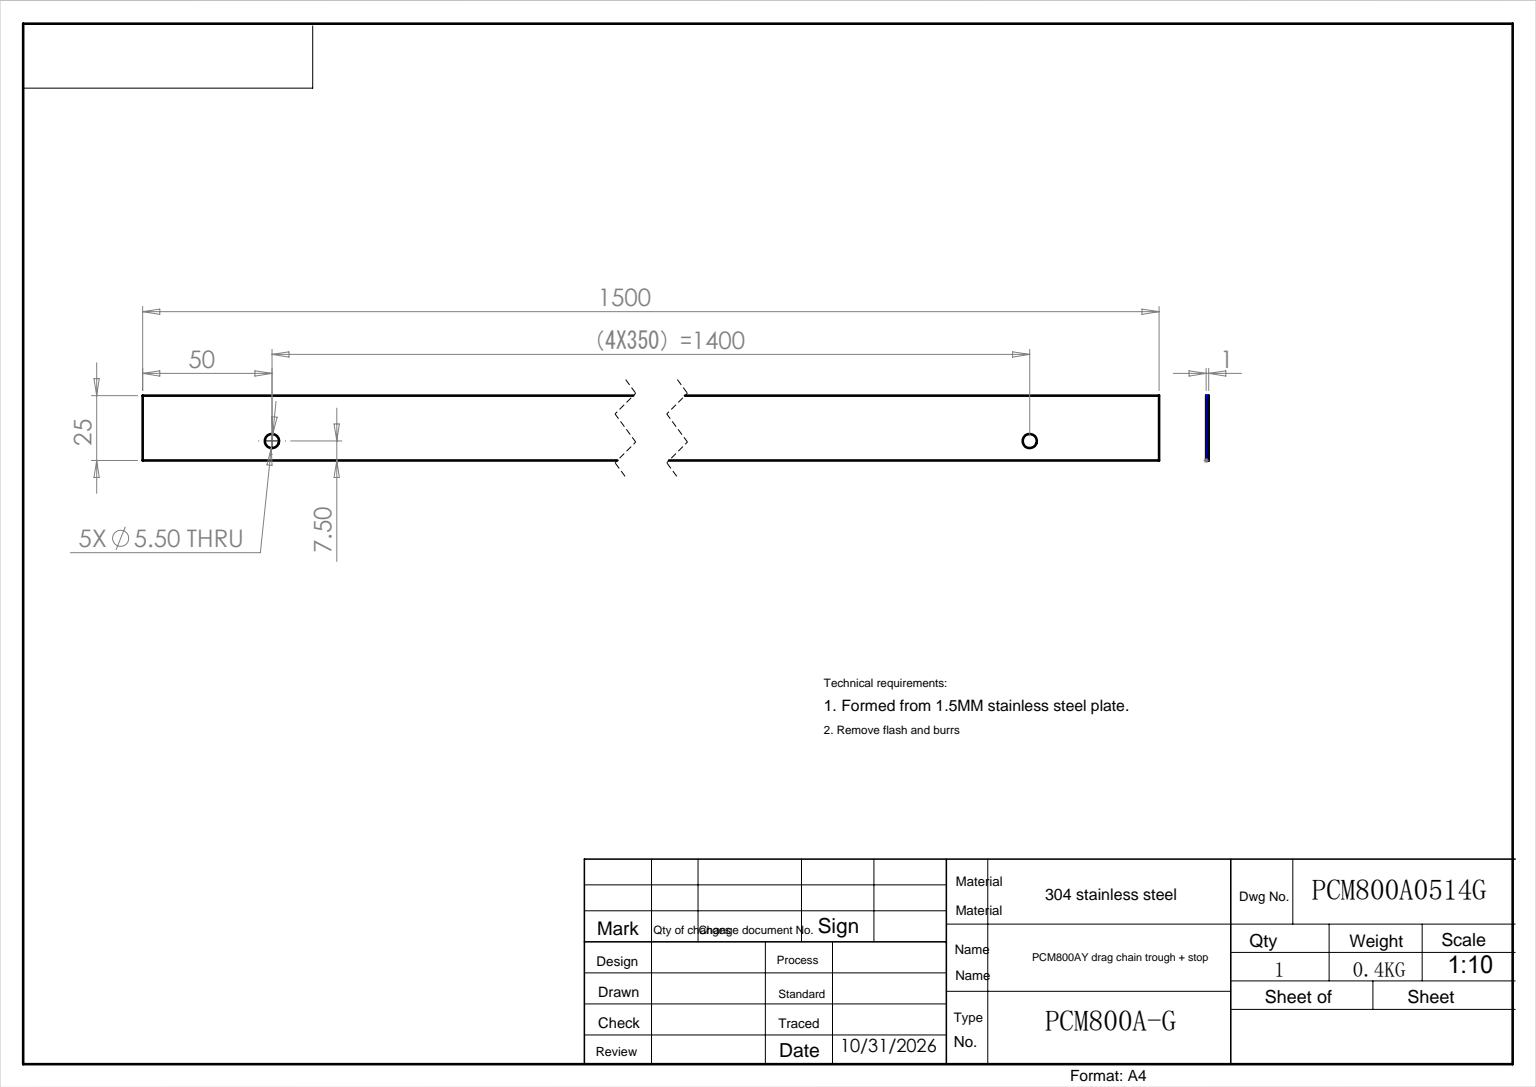
from build123d import *

# Parameters (mm, degrees)
SKETCH_1_W          = 1500
SKETCH_1_H          = 25
EXTRUDE_1_DEPTH     = 1
SKETCH_2_R          = 2.75
CUT_EXTRUDE_1_DEPTH = 10


with BuildPart() as part:
    # 草图1 → 凸台-拉伸1 (new body)
    with BuildSketch(Plane.XY):
        with Locations((750, 12.5)):
            Rectangle(SKETCH_1_W, SKETCH_1_H)
    extrude(amount=EXTRUDE_1_DEPTH)

    # 草图2 → 切除-拉伸1 (cut)
    with BuildSketch(Plane.XY.offset(1)):
        with Locations((50, 7.5)):
            Circle(SKETCH_2_R)
        with Locations((400, 7.5)):
            Circle(SKETCH_2_R)
        with Locations((750, 7.5)):
            Circle(SKETCH_2_R)
        with Locations((1100, 7.5)):
            Circle(SKETCH_2_R)
        with Locations((1450, 7.5)):
            Circle(SKETCH_2_R)
    extrude(amount=-CUT_EXTRUDE_1_DEPTH, mode=Mode.SUBTRACT)


solid = part.part
